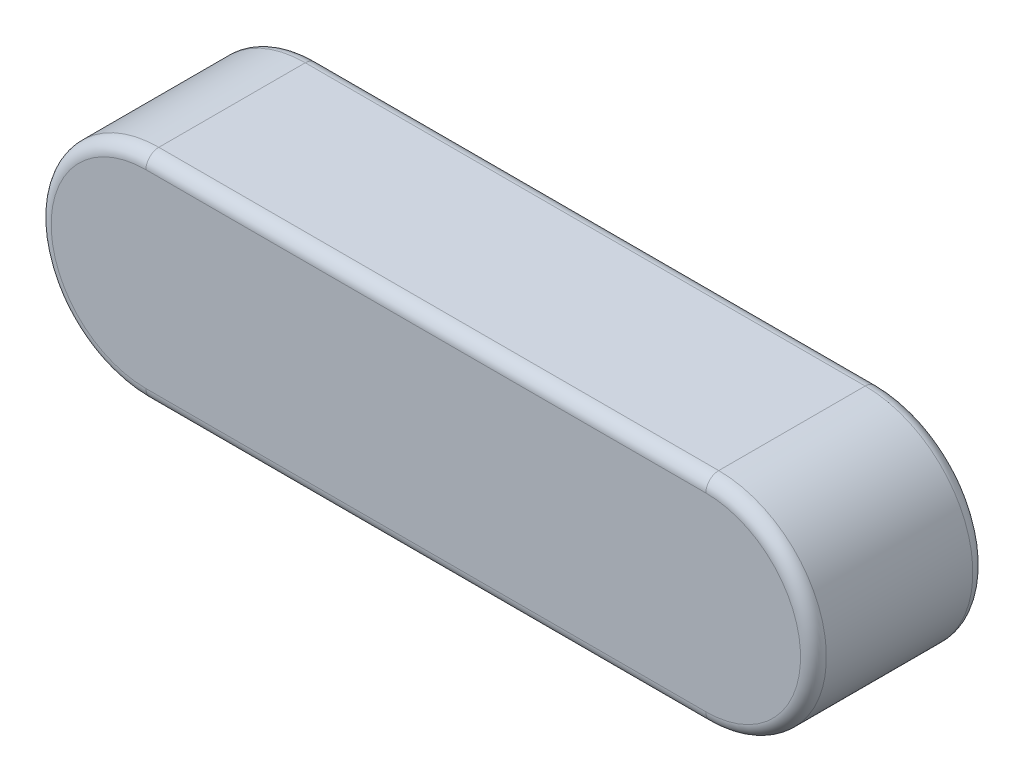
from build123d import *

# Parameters (mm, degrees)
EXTRUDE_512_DEPTH = 8
FILLET_1_R        = 0.6


with BuildPart() as part:
    # 草图1 → Extrude 512 (new body)
    with BuildSketch(Plane.XY):
        with BuildLine():
            Line((-13, 5), (13, 5))
            ThreePointArc((13, 5), (18, 0), (13, -5))
            Line((13, -5), (-13, -5))
            ThreePointArc((-13, -5), (-18, 0), (-13, 5))
        make_face()
    extrude(amount=EXTRUDE_512_DEPTH)

    # 圆角1
    fillet_1_edges = [part.edges().sort_by_distance(p)[0] for p in [
        (18, 0, 8),
        (0, 5, 8),
        (-18, 0, 8),
        (0, 5, 0),
        (18, 0, 0),
        (0, -5, 0),
        (-18, 0, 0),
        (0, -5, 8),
    ]]
    fillet(fillet_1_edges, radius=FILLET_1_R)


solid = part.part
